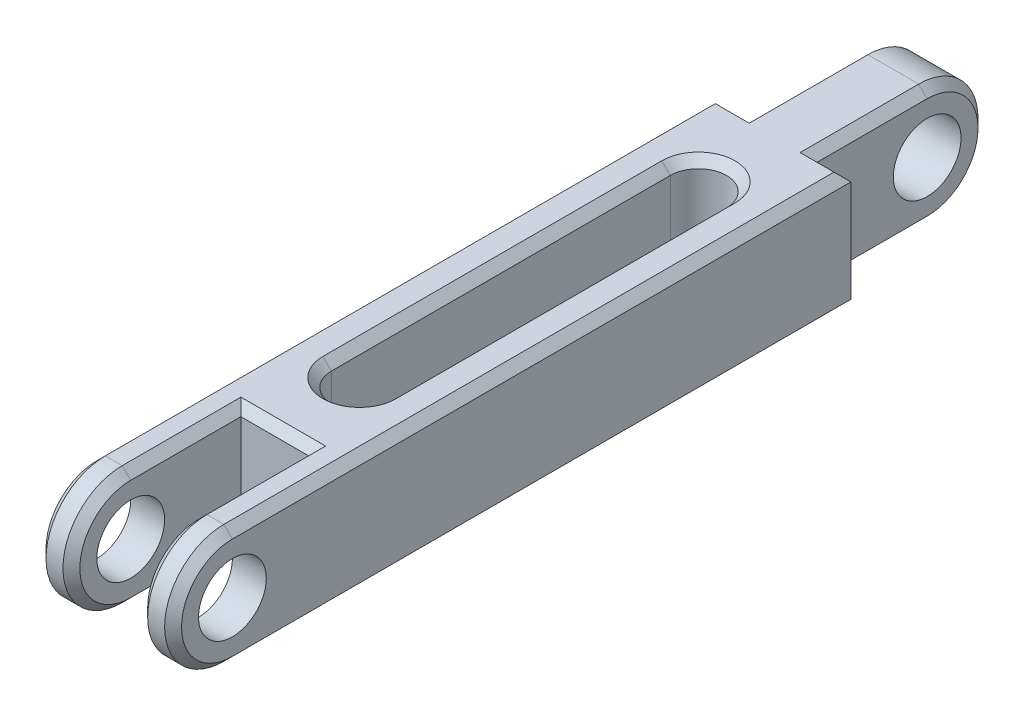
SolidWorks part; units mm, degrees
material "1060 Alloy"
ref_plane "Front Plane" through (0, 0, 0) normal (0, 0, 1) x (1, 0, 0)
ref_plane "Top Plane" through (0, 0, 0) normal (0, 1, 0) x (1, 0, 0)
ref_plane "Right Plane" through (0, 0, 0) normal (1, 0, 0) x (0, 0, -1)
sketch "Sketch1" plane through (0, 0, 0) normal (0, 1, 0) x (1, 0, 0)
  line L0 (4, 40) -> (8, 40)
  line L1 (-8, 40) -> (-4, 40)
  line L2 (-8, 40) -> (-8, -40)
  line L3 (-8, -40) -> (-4, -40)
  line L4 (8, 40) -> (8, -40)
  line L5 (-8, 40) -> (8, -40) construction
  line L6 (-8, -40) -> (8, 40) construction
  line L8 (-4, 40) -> (-4, 60)
  line L9 (-4, 60) -> (4, 60)
  line L10 (4, 40) -> (4, 60)
  line L11 (4, -40) -> (8, -40)
  line L13 (-4, -40) -> (-4, -20)
  line L14 (-4, -20) -> (4, -20)
  line L15 (4, -40) -> (4, -20)
  point P0 (0, 0)
  dimension "D1" = 16
  dimension "D2" = 80
  dimension "D3" = 20
  dimension "D4" = 4
  dimension "D5" = 4
  dimension "D6" = 4
  dimension "D7" = 4
  dimension "D8" = 20
extrude "Boss-Extrude1" add sketch "Sketch1" along normal blind 14
sketch "Sketch2" plane through (4, 0, 0) normal (1, 0, 0) x (0, 0, -1)
  line L0 (60, 14) -> (60, 0) construction
  line L1 (53, 14) -> (60, 14)
  line L2 (60, 14) -> (60, 0)
  line L3 (60, 0) -> (53, 0)
  arc A0 (53, 0) -> (53, 14) centre (53, 7) ccw
  circle A1 centre (53, 7) radius 4
  line M1 (40, 0) -> (60, 0)
  line M2 (60, 0) -> (60, 14)
  line M3 (60, 14) -> (40, 14)
  dimension "D1" = 14
  dimension "D2" = 8
  dimension "D3" = 7
extrude "Cut-Extrude1" cut sketch "Sketch2" against normal blind 14 contours A0 L2 M3 | A0 M1 M2 | A1
sketch "Sketch3" plane through (8, 0, 0) normal (1, 0, 0) x (0, 0, -1)
  line L0 (-40, 14) -> (-40, 0) construction
  line L1 (-33, 14) -> (-40, 14)
  line L2 (-40, 14) -> (-40, 0)
  line L3 (-40, 0) -> (-33, 0)
  arc A0 (-33, 14) -> (-33, 0) centre (-33, 7) ccw
  circle A1 centre (-33, 7) radius 4
  line M1 (-40, 0) -> (40, 0)
  line M3 (40, 14) -> (-40, 14)
  line M4 (-40, 14) -> (-40, 0)
  dimension "D1" = 8
  dimension "D2" = 14
  dimension "D3" = 7
extrude "Cut-Extrude2" cut sketch "Sketch3" against normal blind 30 contours A0 M3 M4 | A0 L2 M1 | A1
sketch "Sketch4" plane through (0, 14, 0) normal (0, 1, 0) x (1, 0, 0)
  line L0 (0, 30) -> (0, -10) construction
  line L1 (3.32, 30) -> (3.32, -10)
  line L2 (-3.32, 30) -> (-3.32, -10)
  line L3 (8, 40) -> (4, 40) construction
  arc A0 (3.32, 30) -> (-3.32, 30) centre (0, 30) ccw
  arc A1 (-3.32, -10) -> (3.32, -10) centre (0, -10) ccw
  point P3 (0, 10)
  dimension "D1" = 40
  dimension "D2" = 10
extrude "Cut-Extrude3" cut sketch "Sketch4" against normal blind 14
chamfer "Chamfer1" distance 1 angle 45 25 edges at (4, 0, -46.5) (8, 0, -3.5) (4, 7, -60) (8, 7, 40) (4, 14, -46.5) (6, 14, -40) (8, 14, -3.5) (4, 0, 26.5) (-4, 0, 26.5) (4, 7, 40) (-4, 7, 40) (4, 14, 26.5) (0, 14, 20) (-4, 14, 26.5) (-4, 0, -46.5) (-8, 0, -3.5) (-4, 7, -60) (-8, 7, 40) (-4, 14, -46.5) (-6, 14, -40) (-8, 14, -3.5) (0, 14, 13.32) (3.32, 14, -10) (0, 14, -33.32) (-3.32, 14, -10)
scale "Scale1" scale about origin uniform scaling yes scale factor 0.5
